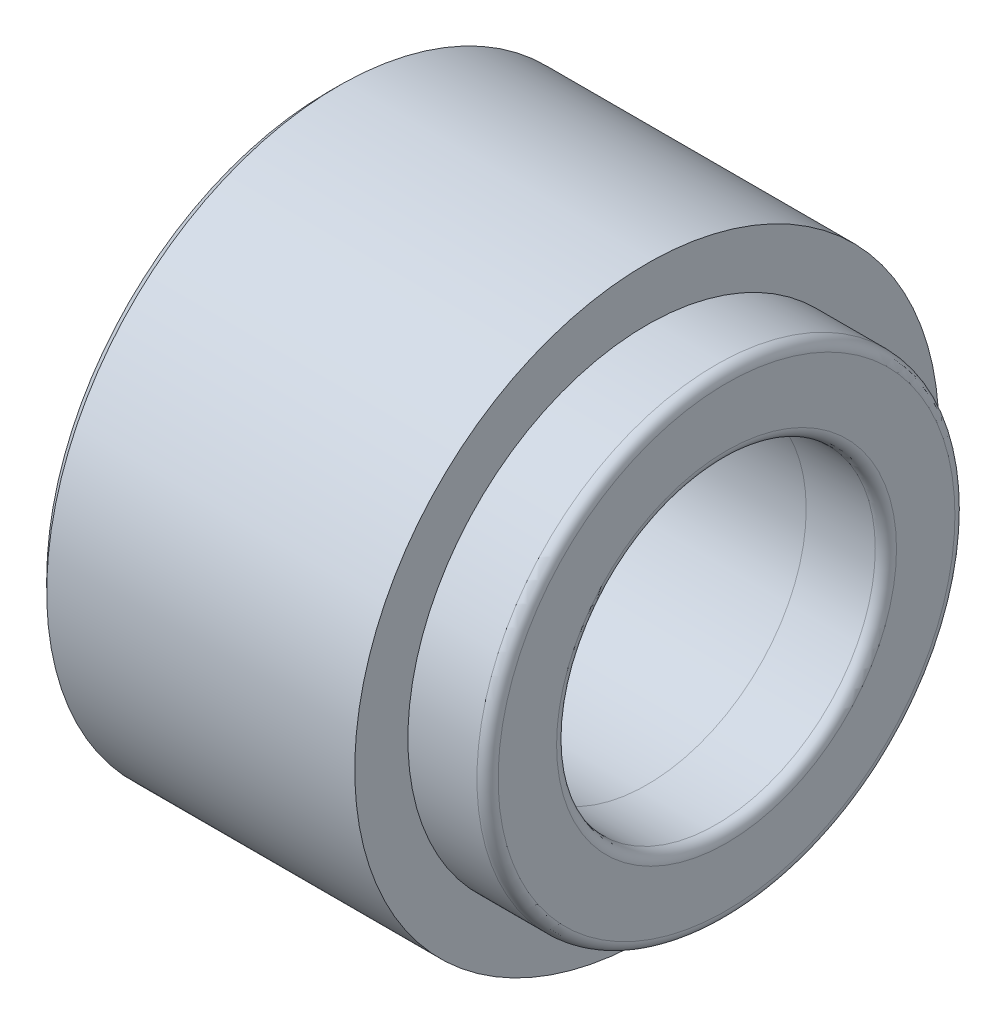
from build123d import *

# Parameters (mm, degrees)
SKETCH_1_R      = 5.5
SKETCH_1_R_2    = 3
EXTRUDE_1_DEPTH = 6
SKETCH_3_R      = 4.5
SKETCH_3_R_2    = 3
EXTRUDE_2_DEPTH = 1.5
FILLET_1_R      = 0.2
CHAMFER_1_SIZE  = 0.2


with BuildPart() as part:
    # 草图1 → 凸台-拉伸1 (new body)
    with BuildSketch(Plane(origin=(0, 0, 0), x_dir=(0, 0, -1), z_dir=(1, 0, 0))):
        Circle(SKETCH_1_R)
        Circle(SKETCH_1_R_2, mode=Mode.SUBTRACT)
    extrude(amount=EXTRUDE_1_DEPTH)

    # 倒角1
    chamfer_1_edges = [part.edges().sort_by_distance(p)[0] for p in [
        (0, 0, 5.5),
        (0, 0, 3),
    ]]
    chamfer(chamfer_1_edges, length=CHAMFER_1_SIZE)


with BuildPart() as body_2:
    # 草图3 → 凸台-拉伸2 (new body)
    with BuildSketch(Plane(origin=(6, 0, 0), x_dir=(0, 0, -1), z_dir=(1, 0, 0))):
        Circle(SKETCH_3_R)
        Circle(SKETCH_3_R_2, mode=Mode.SUBTRACT)
    extrude(amount=EXTRUDE_2_DEPTH)

    # 圆角1
    fillet_1_edges = [body_2.edges().sort_by_distance(p)[0] for p in [
        (7.5, 0, 4.5),
        (7.5, 0, 3),
    ]]
    fillet(fillet_1_edges, radius=FILLET_1_R)


solid = Compound([part.part, body_2.part])
